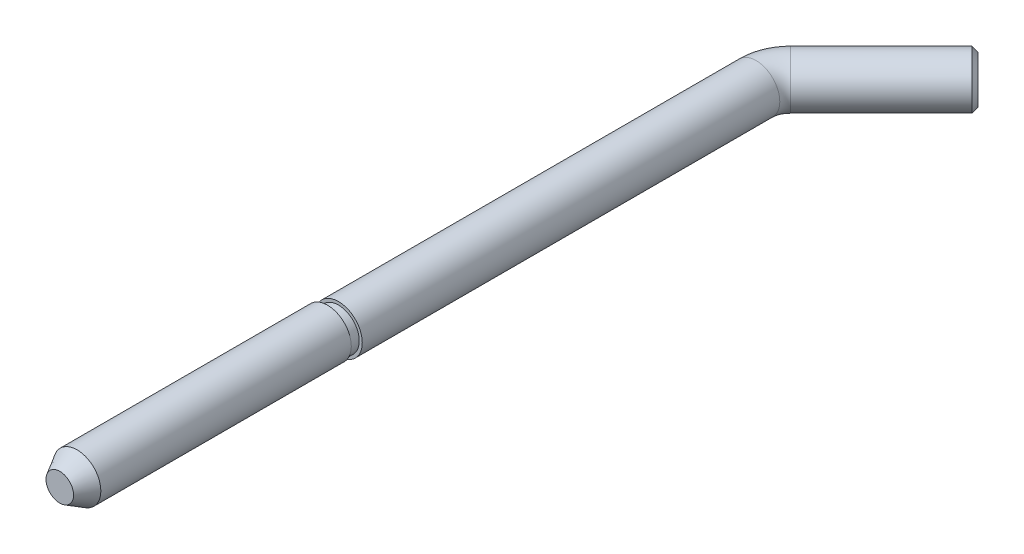
from build123d import *

# Parameters (mm, degrees)
SKETCH1_R           = 2.75
SKETCH4_R           = 2.4
BOSS_EXTRUDE1_DEPTH = 1
SKETCH5_R           = 2.7531
BOSS_EXTRUDE2_DEPTH = 31
CHAMFER2_SIZE       = 2
CHAMFER2_SIZE2      = 1.154700538
CHAMFER3_SIZE       = 0.5


with BuildPart() as part:
    # Sweep1: sweep along a path in Sketch2
    with BuildLine(Plane(origin=(0, 0, 0), x_dir=(1, 0, 0), z_dir=(0, 1, 0))) as sweep1_path:
        Line((0, 0), (0, 48.343145751))
        ThreePointArc((0, 48.343145751), (0.30448187, 49.87387948), (1.171572875, 51.171572875))
        Line((1.171572875, 51.171572875), (12.02081528, 62.02081528))
    # Sketch1 → Sweep1 (sweep)
    with BuildSketch(Plane.XY):
        Circle(SKETCH1_R)
    sweep(path=sweep1_path.line)

    # Sketch4 → Boss-Extrude1 (add)
    with BuildSketch(Plane.XY):
        Circle(SKETCH4_R)
    extrude(amount=BOSS_EXTRUDE1_DEPTH)

    # Sketch5 → Boss-Extrude2 (add)
    with BuildSketch(Plane.XY.offset(1)):
        with Locations((-0.271402, 0)):
            Circle(SKETCH5_R)
    extrude(amount=BOSS_EXTRUDE2_DEPTH)

    # Chamfer2
    chamfer2_edges = [part.edges().sort_by_distance(p)[0] for p in [
        (-3.024502, 0, 32),
    ]]
    chamfer2_side = [part.faces().sort_by_distance(p)[0] for p in [
        (-3.024502, 0, 16.5),
    ]]
    chamfer(chamfer2_edges, length=CHAMFER2_SIZE, length2=CHAMFER2_SIZE2, reference=chamfer2_side[0])

    # Chamfer3
    chamfer3_edges = [part.edges().sort_by_distance(p)[0] for p in [
        (10.076271632, 0, -63.965358928),
    ]]
    chamfer(chamfer3_edges, length=CHAMFER3_SIZE)


solid = part.part
